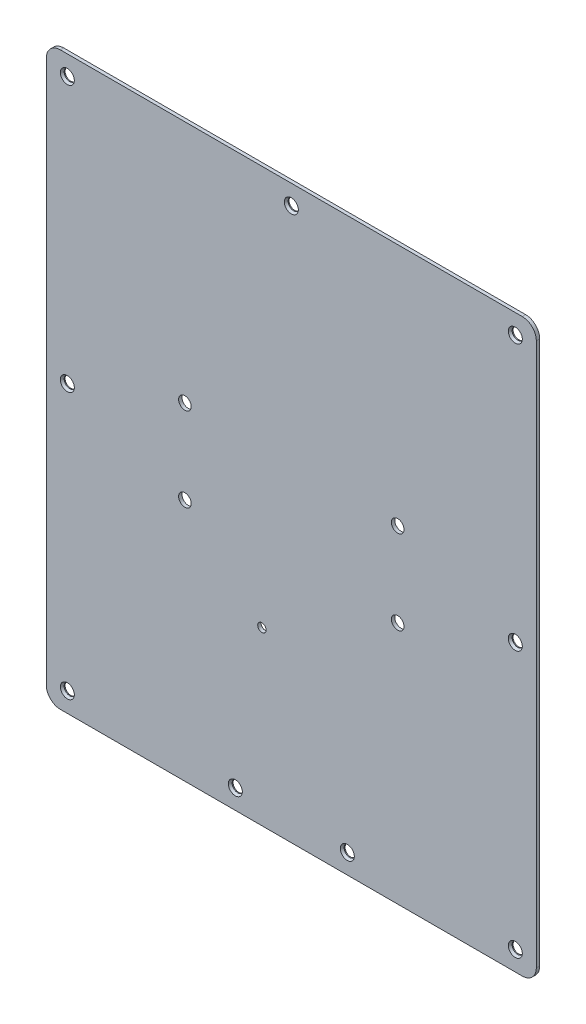
from build123d import *

# Parameters (mm, degrees)
MODEL_R                = 1.5
MODEL_R_2              = 2.25
MODEL_R_3              = 2
BOSS_EXTRUDE1_DEPTH    = 1.2
CHAMFER1_SIZE          = 0.5
CHAMFER1_SIZE2         = 0.866025404
SKETCH2_R              = 1.9
BOSS_EXTRUDE2_DEPTH    = 30
CHAMFER2_SIZE          = 0.5
CHAMFER2_SIZE2         = 0.866025404
CUT_SWEEP1_PITCH       = 1
CUT_SWEEP1_HEIGHT      = 29.25
CUT_SWEEP1_RADIUS      = 1.9
CUT_SWEEP1_START_ANGLE = 180


with BuildPart() as part:
    # Model → Boss-Extrude1 (new body)
    with BuildSketch(Plane.XY):
        with BuildLine():
            Line((-82.5, -102), (82.5, -102))
            ThreePointArc((82.5, -102), (86.035533906, -100.535533906), (87.5, -97))
            Line((87.5, -97), (87.5, 97))
            ThreePointArc((87.5, 97), (86.035533906, 100.535533906), (82.5, 102))
            Line((82.5, 102), (-82.5, 102))
            ThreePointArc((-82.5, 102), (-86.035533906, 100.535533906), (-87.5, 97))
            Line((-87.5, 97), (-87.5, -97))
            ThreePointArc((-87.5, -97), (-86.035533906, -100.535533906), (-82.5, -102))
        make_face()
        with Locations((-10.5, -40.7)):
            Circle(MODEL_R, mode=Mode.SUBTRACT)
        with Locations((-38, -15)):
            Circle(MODEL_R_2, mode=Mode.SUBTRACT)
        with Locations((38, -15)):
            Circle(MODEL_R_2, mode=Mode.SUBTRACT)
        with Locations((-38, 15)):
            Circle(MODEL_R_2, mode=Mode.SUBTRACT)
        with Locations((-80, 95)):
            Circle(MODEL_R_3, mode=Mode.SUBTRACT)
        with Locations((38, 15)):
            Circle(MODEL_R_2, mode=Mode.SUBTRACT)
        with Locations((0, 95)):
            Circle(MODEL_R_3, mode=Mode.SUBTRACT)
        with Locations((80, 95)):
            Circle(MODEL_R_3, mode=Mode.SUBTRACT)
        with Locations((80, 0)):
            Circle(MODEL_R_3, mode=Mode.SUBTRACT)
        with Locations((80, -95)):
            Circle(MODEL_R_3, mode=Mode.SUBTRACT)
        with Locations((20, -95)):
            Circle(MODEL_R_3, mode=Mode.SUBTRACT)
        with Locations((-20, -95)):
            Circle(MODEL_R_3, mode=Mode.SUBTRACT)
        with Locations((-80, -95)):
            Circle(MODEL_R_3, mode=Mode.SUBTRACT)
        with Locations((-80, 0)):
            Circle(MODEL_R_3, mode=Mode.SUBTRACT)
    extrude(amount=BOSS_EXTRUDE1_DEPTH)

    # Chamfer1
    chamfer1_edges = [part.edges().sort_by_distance(p)[0] for p in [
        (-82, 95, 1.2),
        (-2, 95, 1.2),
        (78, 95, 1.2),
        (78, 0, 1.2),
        (-82, 0, 1.2),
        (-82, -95, 1.2),
        (-22, -95, 1.2),
        (18, -95, 1.2),
        (78, -95, 1.2),
    ]]
    chamfer1_side = [part.faces().sort_by_distance(p)[0] for p in [
        (0.002091017, 0.041738462, 1.2),
    ]]
    chamfer(chamfer1_edges, length=CHAMFER1_SIZE, length2=CHAMFER1_SIZE2, reference=chamfer1_side[0])

    # Sketch2 → Boss-Extrude2 (add)
    with BuildSketch(Plane(origin=(0, 0, 0), x_dir=(-1, 0, 0), z_dir=(0, 0, -1))):
        with Locations(Location((0, 0, 0), (0, 0, 180))):
            Circle(SKETCH2_R)
    extrude(amount=BOSS_EXTRUDE2_DEPTH)

    # Chamfer2
    chamfer2_edges = [part.edges().sort_by_distance(p)[0] for p in [
        (-1.9, 0, -30),
    ]]
    chamfer2_side = [part.faces().sort_by_distance(p)[0] for p in [
        (-1.9, 0, -15),
    ]]
    chamfer(chamfer2_edges, length=CHAMFER2_SIZE, length2=CHAMFER2_SIZE2, reference=chamfer2_side[0])

    # Cut-Sweep1: sweep along a helix
    with BuildLine() as cut_sweep1_path:
        add(Helix(CUT_SWEEP1_PITCH, CUT_SWEEP1_HEIGHT, CUT_SWEEP1_RADIUS, center=(0, 0, -30), direction=(0, 0, 1), mode=Mode.PRIVATE).rotate(Axis((0, 0, -30), (0, 0, 1)), CUT_SWEEP1_START_ANGLE))
    # Sketch4 → Cut-Sweep1 (sweep, cut)
    with BuildSketch(Plane(origin=(0, 0, 0), x_dir=(1, 0, 0), z_dir=(0, 1, 0))):
        Polygon((-1.91, 30.4), (-1.91, 29.6), (-1.563589838, 29.8), (-1.563589838, 30.2), align=None)
    sweep(path=cut_sweep1_path.line, is_frenet=True, mode=Mode.SUBTRACT)


solid = part.part
